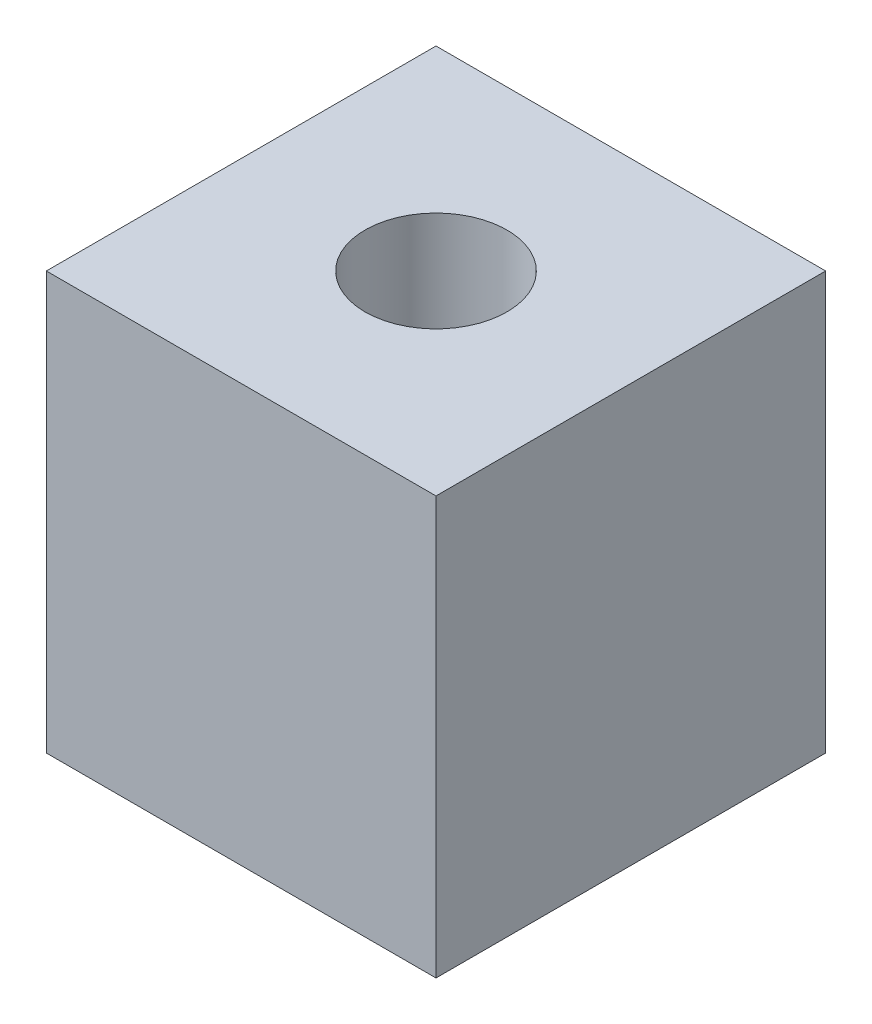
from build123d import *

# Parameters (mm, degrees)
SKETCH1_W           = 28
SKETCH1_H           = 28
SKETCH1_R           = 5
BOSS_EXTRUDE1_DEPTH = 30
M12_TAPPED_HOLE1_D  = 10.2


with BuildPart() as part:
    # Sketch1 → Boss-Extrude1 (new body)
    with BuildSketch(Plane(origin=(0, 0, 0), x_dir=(1, 0, 0), z_dir=(0, 1, 0))):
        Rectangle(SKETCH1_W, SKETCH1_H)
        with Locations(Location((0, 0, 0), (0, 0, 270))):
            Circle(SKETCH1_R, mode=Mode.SUBTRACT)
    extrude(amount=BOSS_EXTRUDE1_DEPTH)

    # M12 Tapped Hole1 (through all)
    with Locations(Plane(origin=(0, 30, 0), x_dir=(1, 0, 0), z_dir=(0, 1, 0))):
        with Locations((0, 0)):
            Hole(M12_TAPPED_HOLE1_D / 2)


solid = part.part
